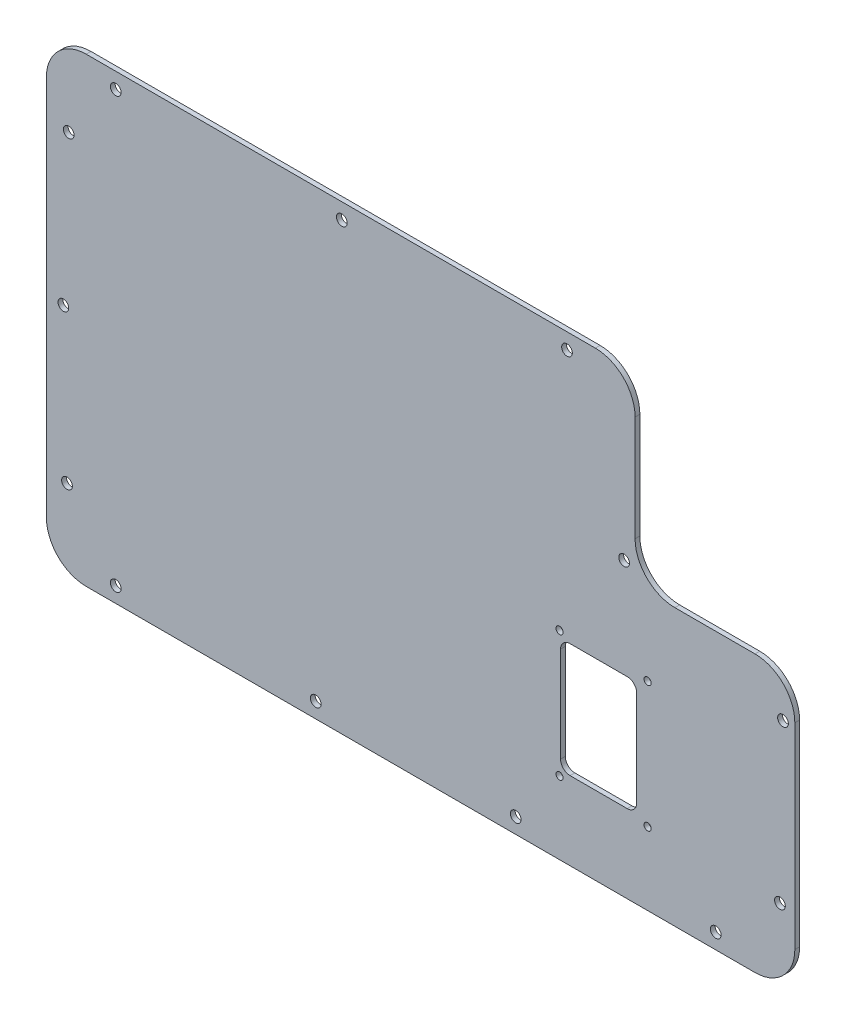
from build123d import *

# Parameters (mm, degrees)
EXTRUDE1_DEPTH                 = 6.35
F_9_16_0_5625_DIAMETER_HOLE1_D = 14.2875
F_3_8_0_375_DIAMETER_HOLE1_D   = 9.525


with BuildPart() as part:
    # Sketch1 → Extrude1 (new body)
    with BuildSketch(Plane.XY):
        with BuildLine():
            Line((0, 53.05662155), (0, 561.62337845))
            ThreePointArc((0, 561.62337845), (15.539924665, 599.140075335), (53.05662155, 614.68))
            Line((53.05662155, 614.68), (731.94337845, 614.68))
            ThreePointArc((731.94337845, 614.68), (769.460075335, 599.140075335), (785, 561.62337845))
            Line((785, 561.62337845), (785, 421.05662155))
            ThreePointArc((785, 421.05662155), (800.539924665, 383.539924665), (838.05662155, 368))
            Line((838.05662155, 368), (944.94337845, 368))
            ThreePointArc((944.94337845, 368), (982.460075335, 352.460075335), (998, 314.94337845))
            Line((998, 314.94337845), (998, 53.05662155))
            ThreePointArc((998, 53.05662155), (982.460075335, 15.539924665), (944.94337845, 0))
            Line((944.94337845, 0), (53.05662155, 0))
            ThreePointArc((53.05662155, 0), (15.539924665, 15.539924665), (0, 53.05662155))
        make_face()
        with BuildLine():
            Line((698.28, 104.14), (774.48, 104.14))
            ThreePointArc((774.48, 104.14), (783.460256121, 107.859743879), (787.18, 116.84))
            Line((787.18, 116.84), (787.18, 243.84))
            ThreePointArc((787.18, 243.84), (783.460256121, 252.820256121), (774.48, 256.54))
            Line((774.48, 256.54), (698.28, 256.54))
            ThreePointArc((698.28, 256.54), (689.299743879, 252.820256121), (685.58, 243.84))
            Line((685.58, 243.84), (685.58, 116.84))
            ThreePointArc((685.58, 116.84), (689.299743879, 107.859743879), (698.28, 104.14))
        make_face(mode=Mode.SUBTRACT)
    extrude(amount=EXTRUDE1_DEPTH)

    # 9/16 (0.5625) Diameter Hole1 (through all)
    with Locations(Plane.XY.offset(6.35)):
        with Locations((22.61, 309.62), (29.72, 512.82), (27.44, 106.42), (92.46, 20.57), (92.46, 593.59), (694.19, 593.59), (393.96, 593.59), (359.16, 20.57), (625.86, 20.57), (892.56, 20.57), (978.16, 96.77), (982.22, 309.62), (770.39, 388.87)):
            Hole(F_9_16_0_5625_DIAMETER_HOLE1_D / 2)

    # 3/8 (0.375) Diameter Hole1 (through all)
    with Locations(Plane.XY.offset(6.35)):
        with Locations((684.28, 264.92), (684.28, 96.77), (801.63, 96.77), (801.63, 264.92)):
            Hole(F_3_8_0_375_DIAMETER_HOLE1_D / 2)


solid = part.part
